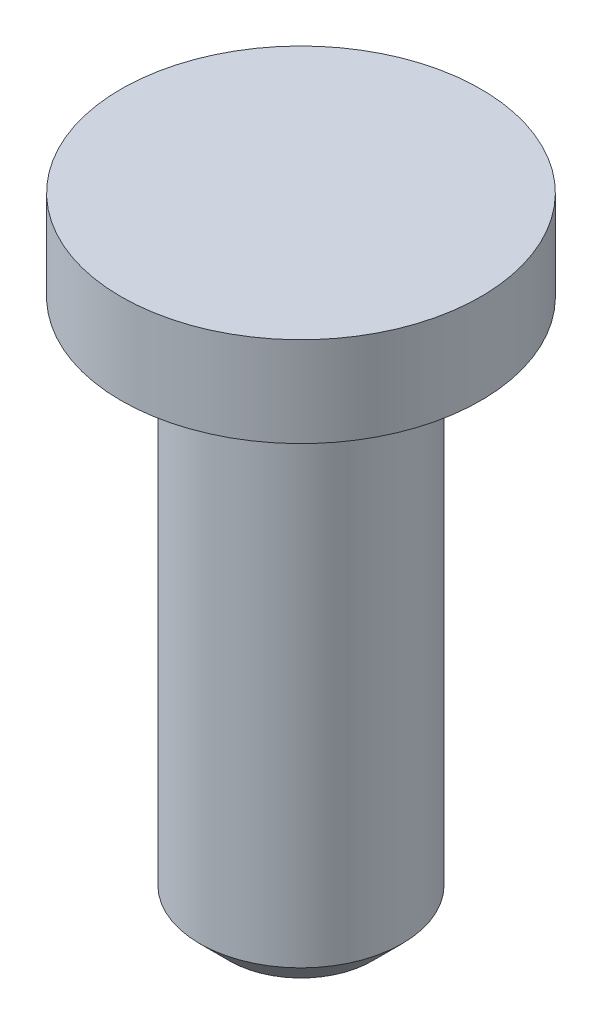
SolidWorks part; units mm, degrees
material "45"
ref_plane "Front Plane" through (0, 0, 0) normal (0, 0, 1) x (1, 0, 0)
ref_plane "Top Plane" through (0, 0, 0) normal (0, 1, 0) x (1, 0, 0)
ref_plane "Right Plane" through (0, 0, 0) normal (1, 0, 0) x (0, 0, -1)
sketch "Sketch1" plane through (0, 0, 0) normal (0, 0, 1) x (1, 0, 0)
  line L0 (-162.3192, -405.8521) -> (-162.3192, -426.8521) construction
  line L2 (-158.9442, -426.8521) -> (-162.3192, -426.8521)
  line L3 (-158.9442, -426.8521) -> (-158.9442, -408.8521)
  line L4 (-158.9442, -408.8521) -> (-156.3192, -408.8521)
  line L7 (-150.3192, -425.1521) -> (-190.0192, -425.1521) construction
  line L9 (-156.3192, -408.8521) -> (-156.3192, -405.8521)
  line L10 (-156.3192, -405.8521) -> (-162.3192, -405.8521)
  line L11 (-162.3192, -405.8521) -> (-162.3192, -426.8521)
  dimension "D1" = 1.7
  dimension "D2" = 18
  dimension "D3" = 3
  dimension "D4" = 12
  dimension "D5" = 6.75
revolve "Revolve2" add sketch "Sketch1" angle 360 about L0
chamfer "Chamfer1" distance 1 angle 45 1 edges at (-162.3192, -426.8521, 3.375)
